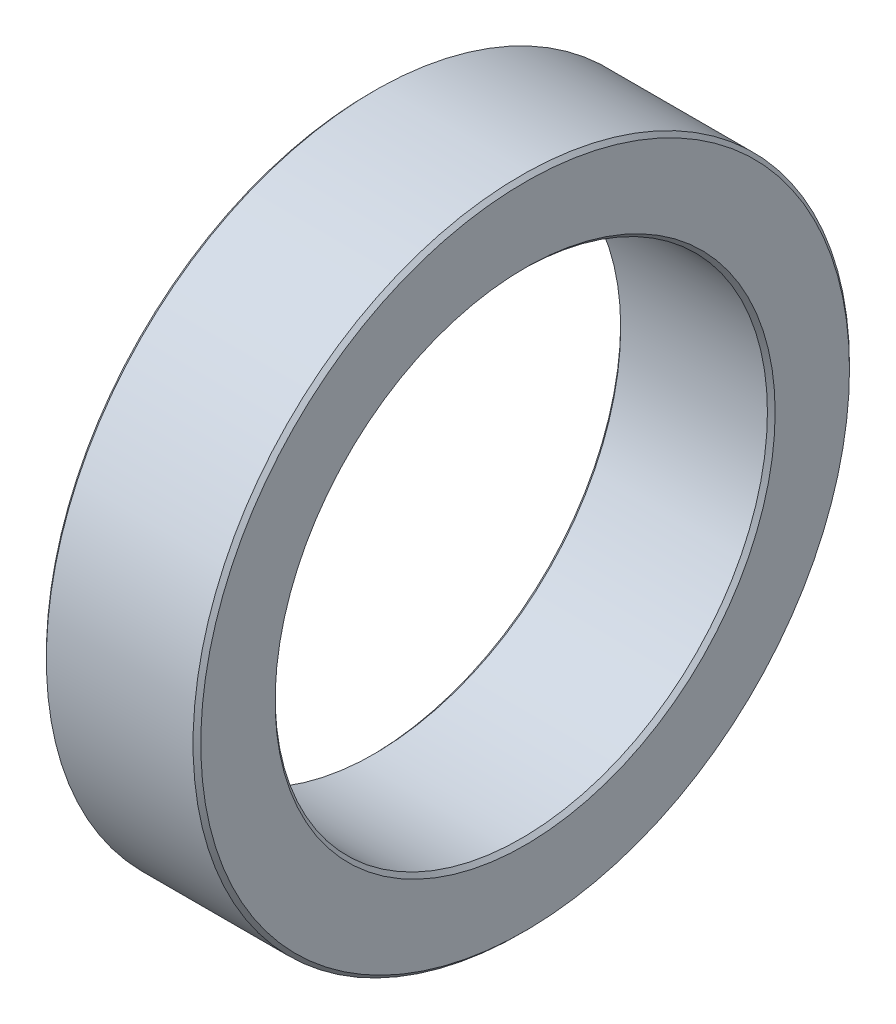
from build123d import *

# Parameters (mm, degrees)
SKETCH1_R           = 17
SKETCH1_R_2         = 12.75
BOSS_EXTRUDE1_DEPTH = 4
CHAMFER1_SIZE       = 0.2


with BuildPart() as part:
    # Sketch1 → Boss-Extrude1 (new, symmetric)
    with BuildSketch(Plane(origin=(0, 0, 0), x_dir=(0, 0, -1), z_dir=(1, 0, 0))):
        Circle(SKETCH1_R)
        Circle(SKETCH1_R_2, mode=Mode.SUBTRACT)
    extrude(amount=BOSS_EXTRUDE1_DEPTH, both=True)

    # Chamfer1
    chamfer1_edges = [part.edges().sort_by_distance(p)[0] for p in [
        (-4, 0, 17),
        (4, 0, 17),
        (-4, 0, 12.75),
        (4, 0, 12.75),
    ]]
    chamfer(chamfer1_edges, length=CHAMFER1_SIZE)


solid = part.part
